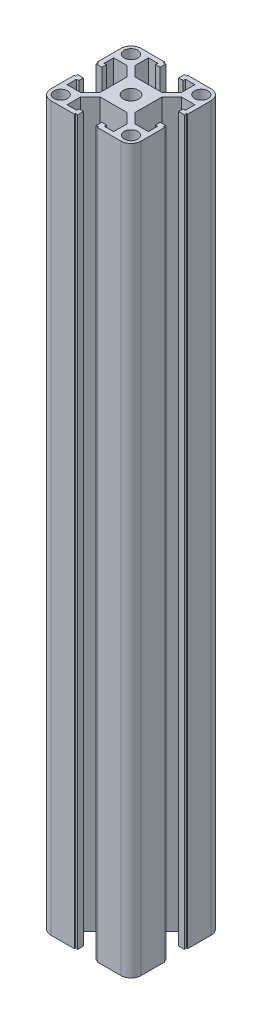
from build123d import *

# Parameters (mm, degrees)
SKETCH16_R     = 3.4
SKETCH16_R_2   = 3
MEMBER_1_DEPTH = 320


with BuildPart() as part:
    # Sketch16 → Member 1 (new body)
    with BuildSketch(Plane(origin=(0, 0, 0), x_dir=(-1, 0, 0), z_dir=(0, 1, 0))):
        with BuildLine():
            Line((-5.1, 20), (-5.1, 19.5))
            Line((-5.1, 19.5), (-4.1, 19.5))
            Line((-4.1, 19.5), (-4.1, 17))
            Line((-4.1, 17), (-6.1, 17))
            Line((-6.1, 17), (-6.1, 18))
            Line((-6.1, 18), (-10.3, 18))
            Line((-10.3, 18), (-10.3, 12))
            Line((-10.3, 12), (-6, 7.7))
            Line((-6, 7.7), (6, 7.7))
            Line((6, 7.7), (10.3, 12))
            Line((10.3, 12), (10.3, 18))
            Line((10.3, 18), (6.1, 18))
            Line((6.1, 18), (6.1, 17))
            Line((6.1, 17), (4.1, 17))
            Line((4.1, 17), (4.1, 19.5))
            Line((4.1, 19.5), (5.1, 19.5))
            Line((5.1, 19.5), (5.1, 20))
            Line((5.1, 20), (15.5, 20))
            ThreePointArc((15.5, 20), (18.681980515, 18.681980515), (20, 15.5))
            Line((20, 15.5), (20, 5.1))
            Line((20, 5.1), (19.5, 5.1))
            Line((19.5, 5.1), (19.5, 4.1))
            Line((19.5, 4.1), (17, 4.1))
            Line((17, 4.1), (17, 6.1))
            Line((17, 6.1), (18, 6.1))
            Line((18, 6.1), (18, 10.3))
            Line((18, 10.3), (12, 10.3))
            Line((12, 10.3), (7.7, 6))
            Line((7.7, 6), (7.7, -6))
            Line((7.7, -6), (12, -10.3))
            Line((12, -10.3), (18, -10.3))
            Line((18, -10.3), (18, -6.1))
            Line((18, -6.1), (17, -6.1))
            Line((17, -6.1), (17, -4.1))
            Line((17, -4.1), (19.5, -4.1))
            Line((19.5, -4.1), (19.5, -5.1))
            Line((19.5, -5.1), (20, -5.1))
            Line((20, -5.1), (20, -15.5))
            ThreePointArc((20, -15.5), (18.681980515, -18.681980515), (15.5, -20))
            Line((15.5, -20), (5.1, -20))
            Line((5.1, -20), (5.1, -19.5))
            Line((5.1, -19.5), (4.1, -19.5))
            Line((4.1, -19.5), (4.1, -17))
            Line((4.1, -17), (6.1, -17))
            Line((6.1, -17), (6.1, -18))
            Line((6.1, -18), (10.3, -18))
            Line((10.3, -18), (10.3, -12))
            Line((10.3, -12), (6, -7.7))
            Line((6, -7.7), (-6, -7.7))
            Line((-6, -7.7), (-10.3, -12))
            Line((-10.3, -12), (-10.3, -18))
            Line((-10.3, -18), (-6.1, -18))
            Line((-6.1, -18), (-6.1, -17))
            Line((-6.1, -17), (-4.1, -17))
            Line((-4.1, -17), (-4.1, -19.5))
            Line((-4.1, -19.5), (-5.1, -19.5))
            Line((-5.1, -19.5), (-5.1, -20))
            Line((-5.1, -20), (-15.5, -20))
            ThreePointArc((-15.5, -20), (-18.681980515, -18.681980515), (-20, -15.5))
            Line((-20, -15.5), (-20, -5.1))
            Line((-20, -5.1), (-19.5, -5.1))
            Line((-19.5, -5.1), (-19.5, -4.1))
            Line((-19.5, -4.1), (-17, -4.1))
            Line((-17, -4.1), (-17, -6.1))
            Line((-17, -6.1), (-18, -6.1))
            Line((-18, -6.1), (-18, -10.3))
            Line((-18, -10.3), (-12, -10.3))
            Line((-12, -10.3), (-7.7, -6))
            Line((-7.7, -6), (-7.7, 6))
            Line((-7.7, 6), (-12, 10.3))
            Line((-12, 10.3), (-18, 10.3))
            Line((-18, 10.3), (-18, 6.1))
            Line((-18, 6.1), (-17, 6.1))
            Line((-17, 6.1), (-17, 4.1))
            Line((-17, 4.1), (-19.5, 4.1))
            Line((-19.5, 4.1), (-19.5, 5.1))
            Line((-19.5, 5.1), (-20, 5.1))
            Line((-20, 5.1), (-20, 15.5))
            ThreePointArc((-20, 15.5), (-18.681980515, 18.681980515), (-15.5, 20))
            Line((-15.5, 20), (-5.1, 20))
        make_face()
        Circle(SKETCH16_R, mode=Mode.SUBTRACT)
        with Locations((-15.556349186, 15.556349186)):
            Circle(SKETCH16_R_2, mode=Mode.SUBTRACT)
        with Locations((15.556349186, 15.556349186)):
            Circle(SKETCH16_R_2, mode=Mode.SUBTRACT)
        with Locations((15.556349186, -15.556349186)):
            Circle(SKETCH16_R_2, mode=Mode.SUBTRACT)
        with Locations((-15.556349186, -15.556349186)):
            Circle(SKETCH16_R_2, mode=Mode.SUBTRACT)
    extrude(amount=MEMBER_1_DEPTH)


solid = part.part
